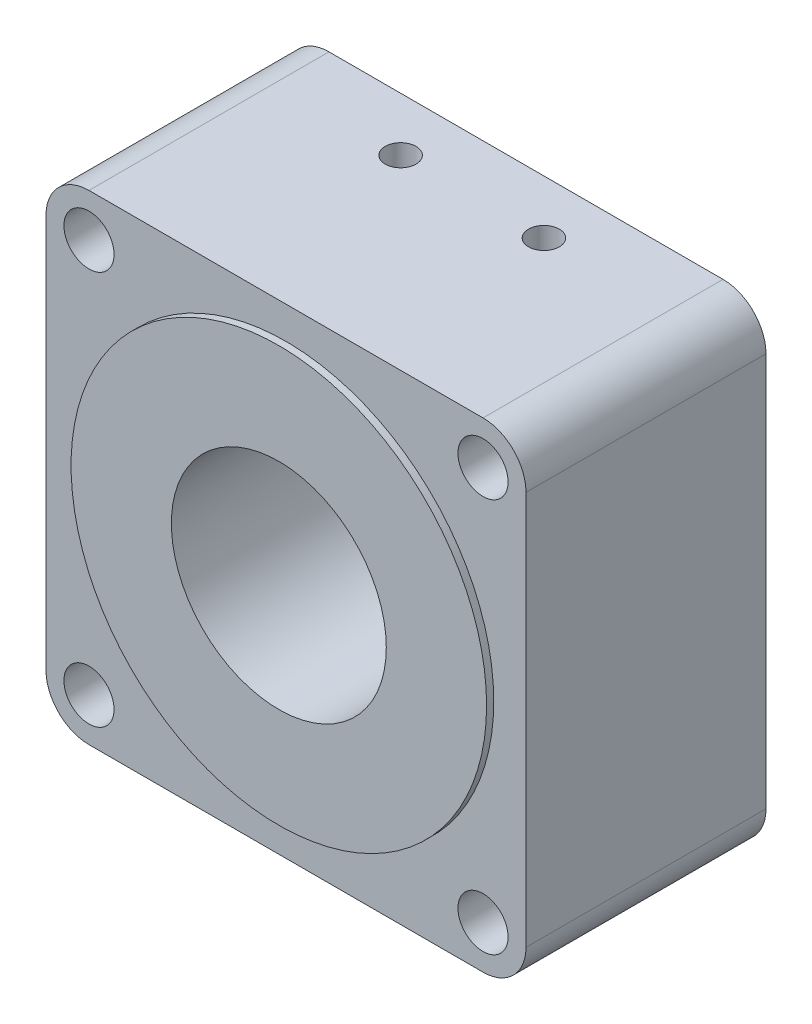
SolidWorks part; units mm, degrees
ref_plane "Front Plane" through (0, 0, 0) normal (0, 0, 1) x (1, 0, 0)
ref_plane "Top Plane" through (0, 0, 0) normal (0, 1, 0) x (1, 0, 0)
ref_plane "Right Plane" through (0, 0, 0) normal (1, 0, 0) x (0, 0, -1)
sketch "Sketch1" plane through (0, 0, 0) normal (0, 0, 1) x (1, 0, 0)
  line L1 (67, 67) -> (-67, 67)
  line L2 (67, 67) -> (67, -67)
  line L3 (67, -67) -> (-67, -67)
  line L4 (-67, 67) -> (-67, -67)
  line L5 (67, 67) -> (-67, -67) construction
  line L6 (67, -67) -> (-67, 67) construction
  point P0 (0, 0)
  dimension "D1" = 134
  dimension "D2" = 134
extrude "Boss-Extrude1" add sketch "Sketch1" along normal blind 67
fillet "Fillet1" radius 12 4 edges at (67, -67, 33.5) (-67, -67, 33.5) (-67, 67, 33.5) (67, 67, 33.5)
sketch "Sketch2" plane through (0, 0, 67) normal (0, 0, 1) x (1, 0, 0)
  circle A0 centre (0, 0) radius 30
  dimension "D1" = 60
extrude "Cut-Extrude1" cut sketch "Sketch2" against normal blind 67
sketch "Sketch3" plane through (0, 0, 67) normal (0, 0, 1) x (1, 0, 0)
  circle A0 centre (0, 0) radius 58
  circle A1 centre (0, 0) radius 30 construction
  circle A2 centre (0, 0) radius 30
  dimension "D1" = 116
extrude "Boss-Extrude2" add sketch "Sketch3" along normal blind 2
sketch "Sketch4" plane through (0, 0, 0) normal (0, 0, -1) x (-1, 0, 0)
  circle A0 centre (0, 0) radius 58
  circle A1 centre (0, 0) radius 30
  circle A2 centre (0, 0) radius 30 construction
  dimension "D1" = 116
extrude "Boss-Extrude3" add sketch "Sketch4" along normal blind 2
sketch "Sketch5" plane through (0, 0, 0) normal (0, 0, -1) x (-1, 0, 0)
  line L1 (55, -55) -> (-55, -55) construction
  line L2 (55, -55) -> (55, 55) construction
  line L3 (55, 55) -> (-55, 55) construction
  line L4 (-55, -55) -> (-55, 55) construction
  line L5 (55, -55) -> (-55, 55) construction
  line L6 (55, 55) -> (-55, -55) construction
  circle A0 centre (-55, 55) radius 7
  circle A1 centre (55, 55) radius 7
  circle A2 centre (55, -55) radius 7
  circle A3 centre (-55, -55) radius 7
  point P0 (0, 0)
  dimension "D3" = 14
  dimension "D1" = 110
  dimension "D2" = 110
extrude "Cut-Extrude2" cut sketch "Sketch5" against normal blind 160
sketch "Sketch6" plane through (0, 0, 0) normal (0, 0, -1) x (-1, 0, 0)
  circle A0 centre (-55, 55) radius 9.5
  circle A1 centre (55, 55) radius 9.5
  circle A2 centre (55, -55) radius 9.5
  circle A3 centre (-55, -55) radius 9.5
  dimension "D1" = 19
extrude "Cut-Extrude3" cut sketch "Sketch6" against normal blind 40
sketch "Sketch7" plane through (0, 0, 0) normal (0, 0, -1) x (-1, 0, 0)
  line L1 (36.71, -52.425) -> (-36.71, -52.425) construction
  line L2 (36.71, -52.425) -> (36.71, 52.425) construction
  line L3 (36.71, 52.425) -> (-36.71, 52.425) construction
  line L4 (-36.71, -52.425) -> (-36.71, 52.425) construction
  line L5 (36.71, -52.425) -> (-36.71, 52.425) construction
  line L6 (36.71, 52.425) -> (-36.71, -52.425) construction
  circle A0 centre (-36.71, 52.425) radius 4
  circle A1 centre (36.71, 52.425) radius 4
  circle A2 centre (36.71, -52.425) radius 4
  circle A3 centre (-36.71, -52.425) radius 4
  point P0 (0, 0)
  dimension "D3" = 8
  dimension "D1" = 73.42
  dimension "D2" = 104.85
hole_wizard "Size mm Dowel hole 1" positions "Sketch8" profile "Sketch9" hole size "Ø5.0" standard "GB"
sketch "Sketch8" plane through (0, 0, 0) normal (0, 0, -1) x (-1, 0, 0)
  point P0 (-36.71, 52.425)
  point P3 (36.71, 52.425)
  point P6 (36.71, -52.425)
  point P9 (-36.71, -52.425)
sketch "Sketch9" plane through (36.71, 52.425, 0) normal (1, 0, 0) x (0, 1, 0)
  line L0 (0, 0) -> (0, 27.0537)
  line L1 (0, 27.0537) -> (4.25, 24.5)
  line L2 (4.25, 24.5) -> (4.25, 0)
  line L5 (4.25, 0) -> (0, 0)
  line L10 (0, 27.0537) -> (-4.25, 24.5) construction
  line L11 (0, -6.35) -> (0, 107.95) construction
  dimension "孔直径" = 8.5
  dimension "孔深度" = 24.5
  dimension "导头角度" = 118
sketch "Sketch10" plane through (0, 0, 0) normal (0, 0, -1) x (-1, 0, 0)
  line L1 (52.425, -36.71) -> (-52.425, -36.71)
  line L2 (52.425, -36.71) -> (52.425, 36.71)
  line L3 (52.425, 36.71) -> (-52.425, 36.71)
  line L4 (-52.425, -36.71) -> (-52.425, 36.71) construction
  line L5 (52.425, -36.71) -> (-52.425, 36.71) construction
  line L6 (52.425, 36.71) -> (-52.425, -36.71) construction
  circle A0 centre (-52.425, 36.71) radius 4
  circle A1 centre (-52.425, -36.71) radius 4
  circle A2 centre (52.425, 36.71) radius 4
  circle A3 centre (52.425, -36.71) radius 4
  point P0 (0, 0)
  dimension "D3" = 8
  dimension "D1" = 73.42
  dimension "D2" = 104.85
hole_wizard "Size mm Dowel hole 2" positions "Sketch11" profile "Sketch12" hole size "Ø5.0" standard "GB"
sketch "Sketch11" plane through (0, 0, 0) normal (0, 0, -1) x (-1, 0, 0)
  point P0 (-52.425, 36.71)
  point P3 (52.425, 36.71)
  point P6 (52.425, -36.71)
  point P9 (-52.425, -36.71)
sketch "Sketch12" plane through (52.425, 36.71, 0) normal (1, 0, 0) x (0, 1, 0)
  line L0 (0, 0) -> (0, 27.0537)
  line L1 (0, 27.0537) -> (4.25, 24.5)
  line L2 (4.25, 24.5) -> (4.25, 0)
  line L5 (4.25, 0) -> (0, 0)
  line L10 (0, 27.0537) -> (-4.25, 24.5) construction
  line L11 (0, -6.35) -> (0, 107.95) construction
  dimension "孔直径" = 8.5
  dimension "孔深度" = 24.5
  dimension "导头角度" = 118
sketch "Sketch13" plane through (0, 67, 0) normal (0, 1, 0) x (1, 0, 0)
  line L0 (55, 0) -> (-55, 0) construction
  circle A0 centre (20, -15) radius 7.4755
  circle A1 centre (-20, -15) radius 6.246
  dimension "D1" = 40
  dimension "D2" = 15
  dimension "D3" = 20
hole_wizard "Size mm Dowel hole 3" positions "Sketch16" profile "Sketch17" hole size "Ø5.0" standard "GB"
sketch "Sketch16" plane through (0, 67, 0) normal (0, 1, 0) x (1, 0, 0)
  point P0 (-20, -15)
  point P3 (20, -15)
sketch "Sketch17" plane through (-20, 67, 15) normal (1, 0, 0) x (0, 0, 1)
  line L0 (0, 0) -> (0, 12.5837)
  line L1 (0, 12.5837) -> (4.3, 10)
  line L2 (4.3, 10) -> (4.3, 0)
  line L5 (4.3, 0) -> (0, 0)
  line L10 (0, 12.5837) -> (-4.3, 10) construction
  line L11 (0, -6.35) -> (0, 107.95) construction
  dimension "孔直径" = 8.6
  dimension "孔深度" = 10
  dimension "导头角度" = 118
